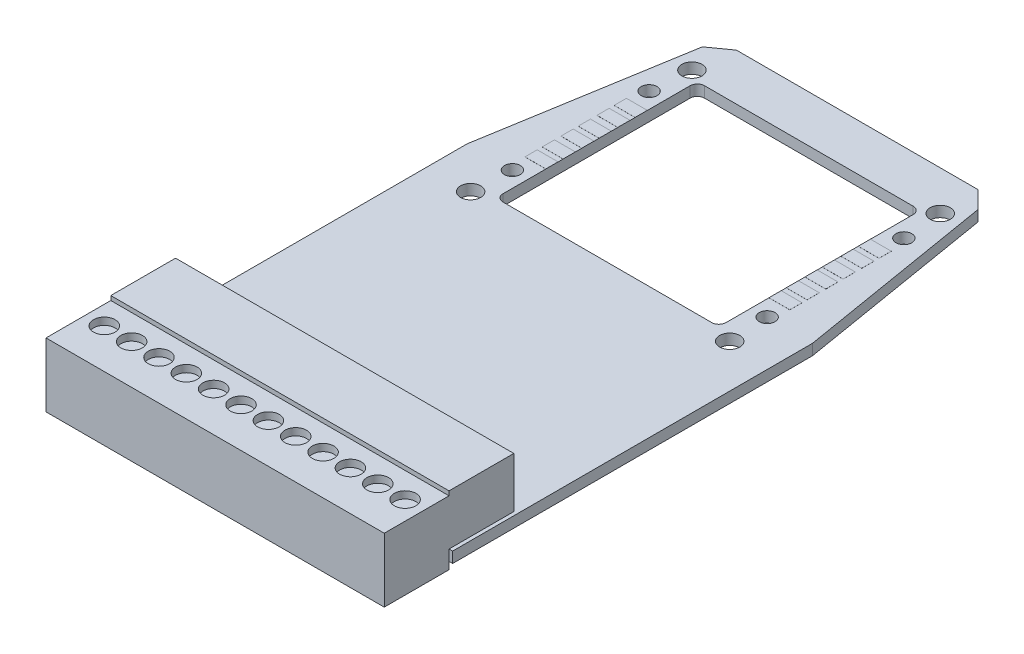
SolidWorks part; units mm, degrees
ref_plane "Front Plane" through (0, 0, 0) normal (0, 0, 1) x (1, 0, 0)
ref_plane "Top Plane" through (0, 0, 0) normal (0, 1, 0) x (1, 0, 0)
ref_plane "Right Plane" through (0, 0, 0) normal (1, 0, 0) x (0, 0, -1)
sketch "Sketch1" plane through (0, 0, 0) normal (0, 1, 0) x (1, 0, 0)
  line L1 (-24, 40) -> (24, 40)
  line L2 (-24, 40) -> (-24, -40)
  line L3 (-24, -40) -> (24, -40)
  line L4 (24, 40) -> (24, -40)
  line L5 (-24, 40) -> (24, -40) construction
  line L6 (-24, -40) -> (24, 40) construction
  point P0 (0, 0)
  dimension "D1" = 48
  dimension "D2" = 80
extrude "Boss-Extrude1" add sketch "Sketch1" along normal mid plane 1.5
sketch "Sketch2" plane through (0, 0.75, 0) normal (0, 1, 0) x (1, 0, 0)
  line L0 (-19, 40) -> (-24, 40)
  line L1 (-24, 40) -> (-24, 10)
  line L2 (-24, 10) -> (-19, 40)
  line L3 (19, 40) -> (24, 40)
  line L4 (24, 40) -> (24, 10)
  line L5 (24, 10) -> (19, 40)
  line L6 (24, 40) -> (-24, 40) construction
  line L7 (-24, 40) -> (-24, -40) construction
  line L8 (24, -40) -> (24, 40) construction
  line L9 (0, 0) -> (0, 47.1853) construction
  dimension "D1" = 30
  dimension "D2" = 38
extrude "Cut-Extrude1" cut sketch "Sketch2" against normal through all
sketch "Sketch3" plane through (0, 0.75, 0) normal (0, 1, 0) x (1, 0, 0)
  line L0 (0, 0) -> (0, 45.0424) construction
  line L1 (15.5, 33.5) -> (-15.5, 33.5)
  line L2 (15.5, 33.5) -> (15.5, 5.5)
  line L3 (15.5, 5.5) -> (-15.5, 5.5)
  line L4 (-15.5, 33.5) -> (-15.5, 5.5)
  line L5 (19, 40) -> (-19, 40) construction
  dimension "D1" = 6.5
  dimension "D2" = 28
  dimension "D3" = 31
extrude "Cut-Extrude2" cut sketch "Sketch3" against normal through all
fillet "Fillet1" radius 1 4 edges at (-15.5, 0, -5.5) (15.5, 0, -5.5) (15.5, 0, -33.5) (-15.5, 0, -33.5)
hole_wizard "Ø2.8 (2.8) Diameter Hole1" positions "Sketch5" profile "Sketch4" hole size "Ø2.8" standard "Gb" end condition through all
sketch "Sketch5" plane through (0, 0.75, 0) normal (0, 1, 0) x (1, 0, 0)
  line L0 (0, 0) -> (0, 41.5288) construction
  line L2 (19, 40) -> (-19, 40) construction
  point P0 (17.25, 34.5)
  point P3 (18, 4.5)
  point P6 (-17.25, 34.5)
  point P9 (-18, 4.5)
  dimension "D1" = 34.5
  dimension "D2" = 36
  dimension "D3" = 30
  dimension "D4" = 5.5
sketch "Sketch4" plane through (17.25, 0.75, -34.5) normal (1, 0, 0) x (0, 0, 1)
  line L0 (0, 0) -> (0, 1.5)
  line L1 (0, 1.5) -> (1.4, 1.5)
  line L2 (1.4, 1.5) -> (1.4, 0)
  line L5 (1.4, 0) -> (0, 0)
  line L11 (0, -6.35) -> (0, 107.95) construction
  dimension "通孔孔直径" = 2.8
  dimension "通孔孔深度" = 1.5
hole_wizard "Ø2.2 (2.2) Diameter Hole1" positions "Sketch7" profile "Sketch6" hole size "Ø2.2" standard "Gb" end condition through all
sketch "Sketch7" plane through (0, 0.75, 0) normal (0, 1, 0) x (1, 0, 0)
  line L0 (0, 0) -> (0, 36.6946) construction
  line L2 (19, 40) -> (-19, 40) construction
  point P0 (17.7, 29)
  point P3 (17.7, 10)
  point P6 (-17.7, 10)
  point P9 (-17.7, 29)
  dimension "D1" = 35.4
  dimension "D2" = 19
  dimension "D3" = 11
sketch "Sketch6" plane through (17.7, 0.75, -29) normal (1, 0, 0) x (0, 0, 1)
  line L0 (0, 0) -> (0, 1.5)
  line L1 (0, 1.5) -> (1.1, 1.5)
  line L2 (1.1, 1.5) -> (1.1, 0)
  line L5 (1.1, 0) -> (0, 0)
  line L11 (0, -6.35) -> (0, 107.95) construction
  dimension "通孔孔直径" = 2.2
  dimension "通孔孔深度" = 1.5
sketch "Sketch8" plane through (0, 0.75, 0) normal (0, 1, 0) x (1, 0, 0)
  line L0 (-24, -40) -> (24, -40) construction
  line L1 (-23.5, -40) -> (23.5, -40)
  line L2 (-23.5, -40) -> (-23.5, -31)
  line L3 (-23.5, -31) -> (23.5, -31)
  line L4 (23.5, -40) -> (23.5, -31)
  line L5 (0, 0) -> (0, -35.7955) construction
  dimension "D1" = 47
  dimension "D2" = 9
extrude "Boss-Extrude2" add sketch "Sketch8" along normal blind 7
sketch "Sketch9" plane through (0, 0, 40) normal (0, 0, 1) x (1, 0, 0)
  line L0 (-23.5, 7.75) -> (-23.5, 0.75) construction
  line L1 (-23.5, -1.75) -> (23.5, -1.75)
  line L2 (-23.5, -1.75) -> (-23.5, 7.15)
  line L3 (-23.5, 7.15) -> (23.5, 7.15)
  line L4 (23.5, -1.75) -> (23.5, 7.15)
  line L5 (23.5, 7.75) -> (23.5, 0.75) construction
  line L7 (-23.5, 7.75) -> (23.5, 7.75) construction
  line L8 (-24, -0.75) -> (24, -0.75) construction
  dimension "D1" = 0.6
  dimension "D2" = 1
extrude "Boss-Extrude3" add sketch "Sketch9" along normal blind 9
sketch "Sketch10" plane through (0, 7.15, 0) normal (0, 1, 0) x (1, 0, 0)
  line L0 (23.5, -49) -> (-23.5, -49) construction
  line L1 (-23.5, -49) -> (-23.5, -40) construction
  circle A0 centre (-20.9, -43.5) radius 1.5
  dimension "D1" = 3
  dimension "D2" = 5.5
  dimension "D3" = 2.6
extrude "Cut-Extrude3" cut sketch "Sketch10" against normal blind 1
pattern_linear "LPattern1" count 12 spacing 3.8 along (1, 0, 0) of "Cut-Extrude3"
sketch "Sketch11" plane through (0, 0.75, 0) normal (0, 1, 0) x (1, 0, 0)
  line L1 (-15.5, 22.45) -> (-18.4, 22.45)
  line L2 (18.4, 24.85) -> (15.5, 24.85)
  line L3 (18.4, 24.85) -> (18.4, 26.55)
  line L4 (18.4, 26.55) -> (15.5, 26.55)
  line L5 (-15.5, 22.45) -> (-15.5, 24.15)
  line L6 (-15.5, 24.15) -> (-18.4, 24.15)
  line L7 (-18.4, 24.85) -> (-15.5, 24.85)
  line L8 (-18.4, 24.85) -> (-18.4, 26.55)
  line L9 (-18.4, 26.55) -> (-15.5, 26.55)
  line L10 (-15.5, 24.85) -> (-15.5, 26.55)
  line L11 (-18.4, 22.45) -> (-18.4, 24.15)
  line L12 (15.5, 24.85) -> (15.5, 26.55)
  line L13 (15.5, 22.45) -> (18.4, 22.45)
  line L14 (14.5, 33.5) -> (-14.5, 33.5) construction
  line L15 (-15.5, 32.5) -> (-15.5, 6.5) construction
  line L16 (15.5, 6.5) -> (15.5, 32.5) construction
  line L17 (15.5, 22.45) -> (15.5, 24.15)
  line L18 (15.5, 24.15) -> (18.4, 24.15)
  line L19 (18.4, 22.45) -> (18.4, 24.15)
  dimension "D1" = 6.95
  dimension "D2" = 1.7
  dimension "D3" = 2.9
  dimension "D4" = 2.9
  dimension "D5" = 1.7
  dimension "D6" = 2.4
extrude "Boss-Extrude4" add sketch "Sketch11" along normal blind 0.01
pattern_linear "LPattern2" count 3 spacing 5 along (0, 0, 1) of "Boss-Extrude4"
chamfer "Chamfer1" distance 2 angle 45 2 edges at (-19, 0, -40) (19, 0, -40)
